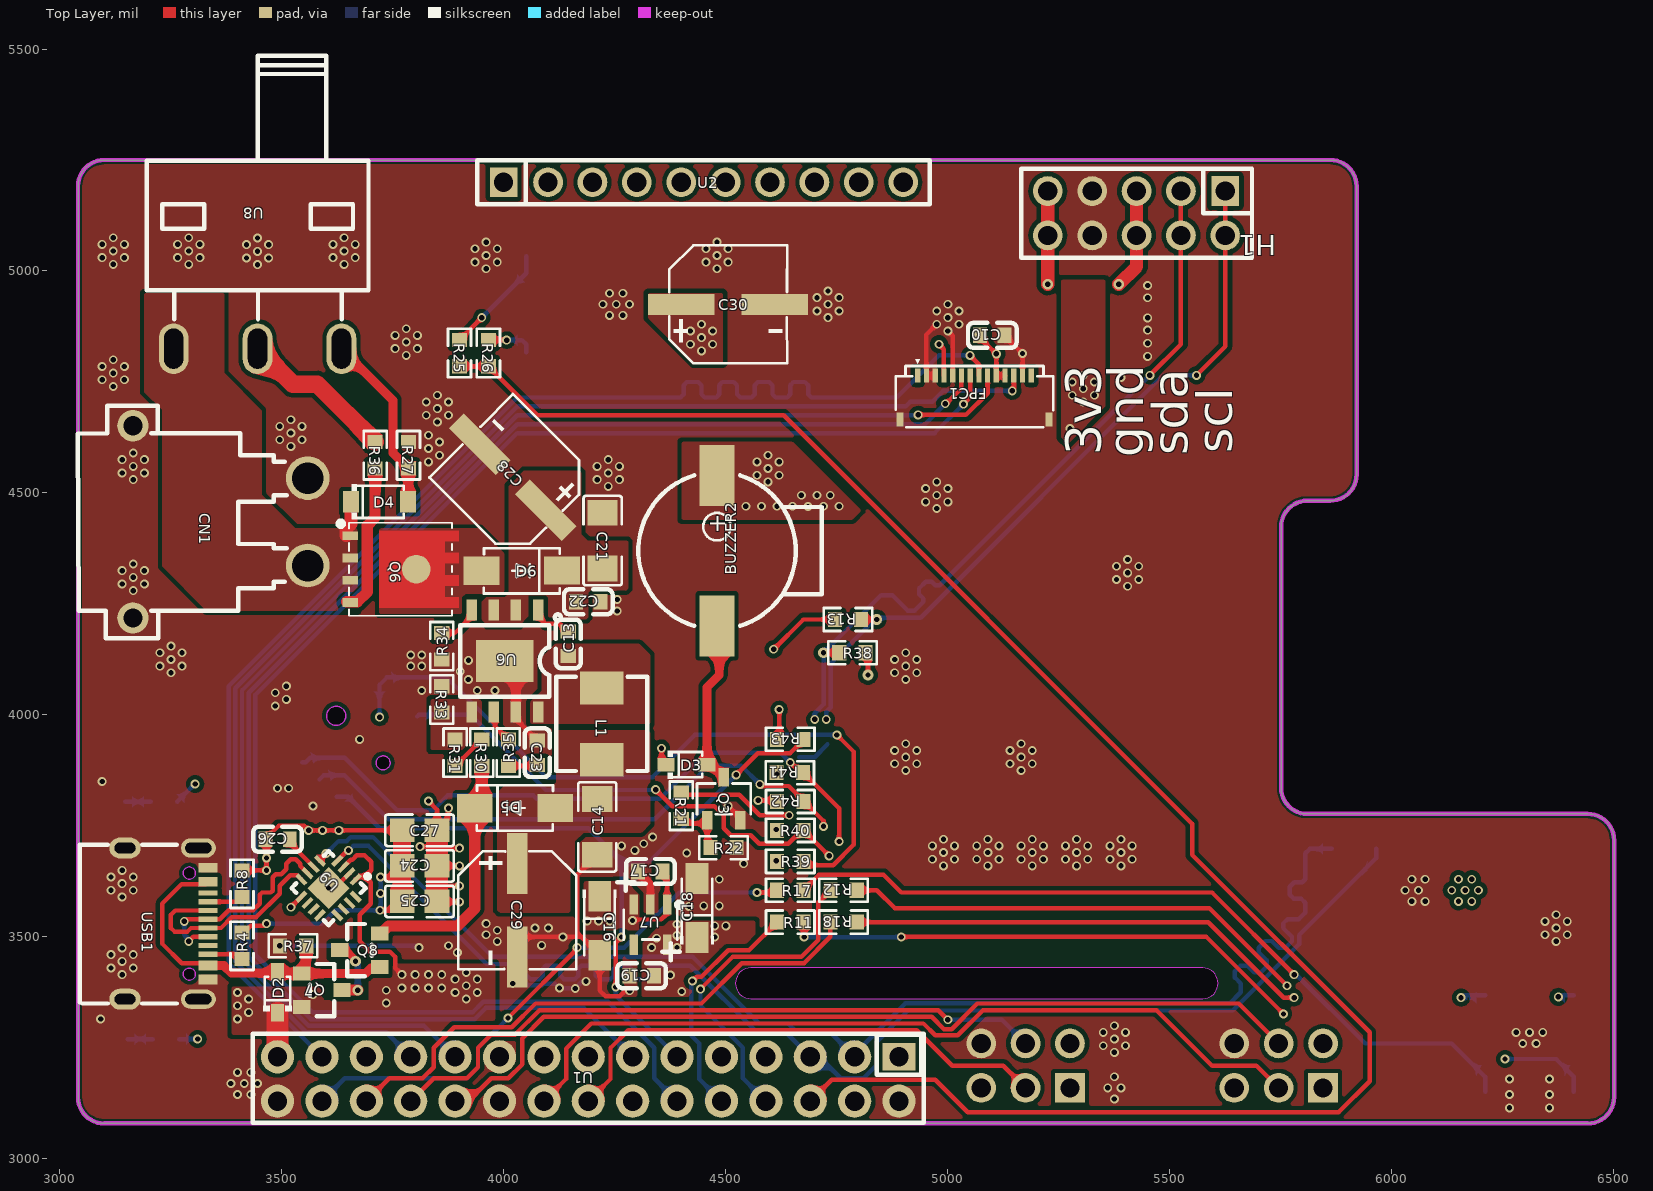
[diagram p0: Top Layer view]
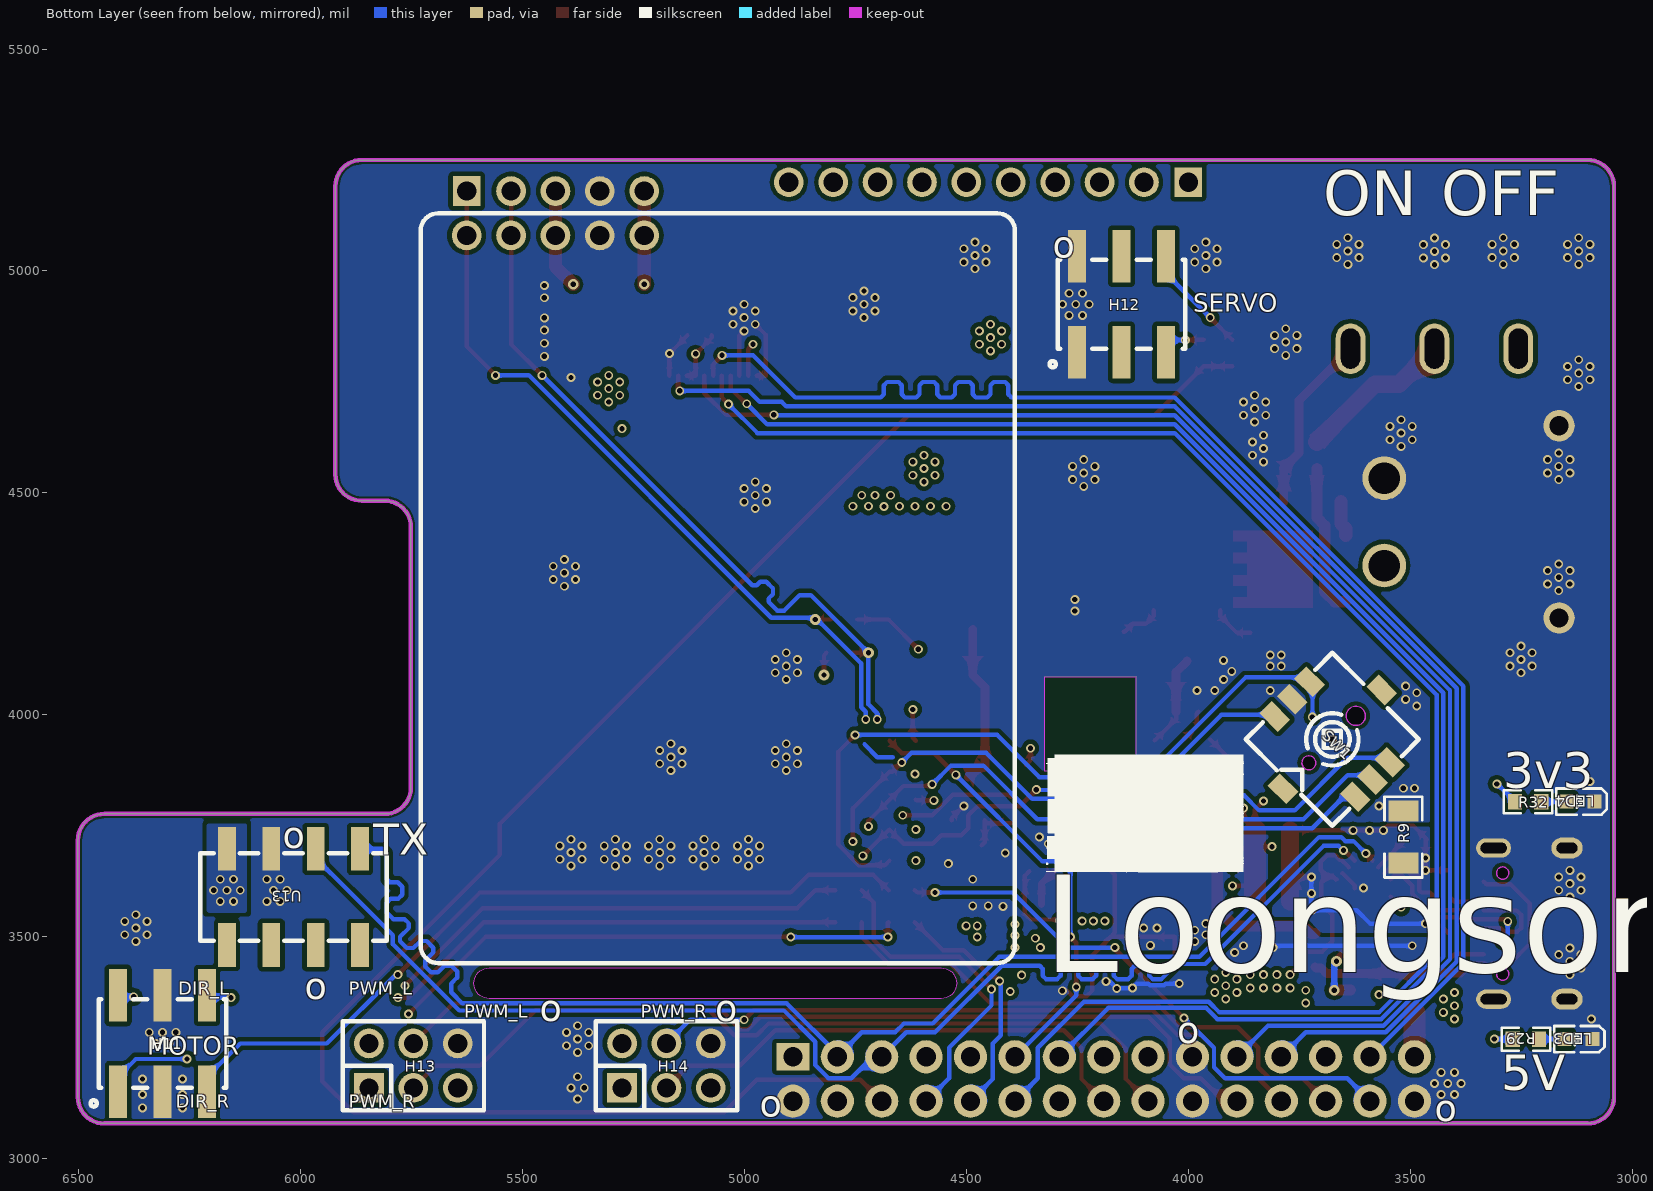
[diagram p1: Bottom Layer view, seen from below]
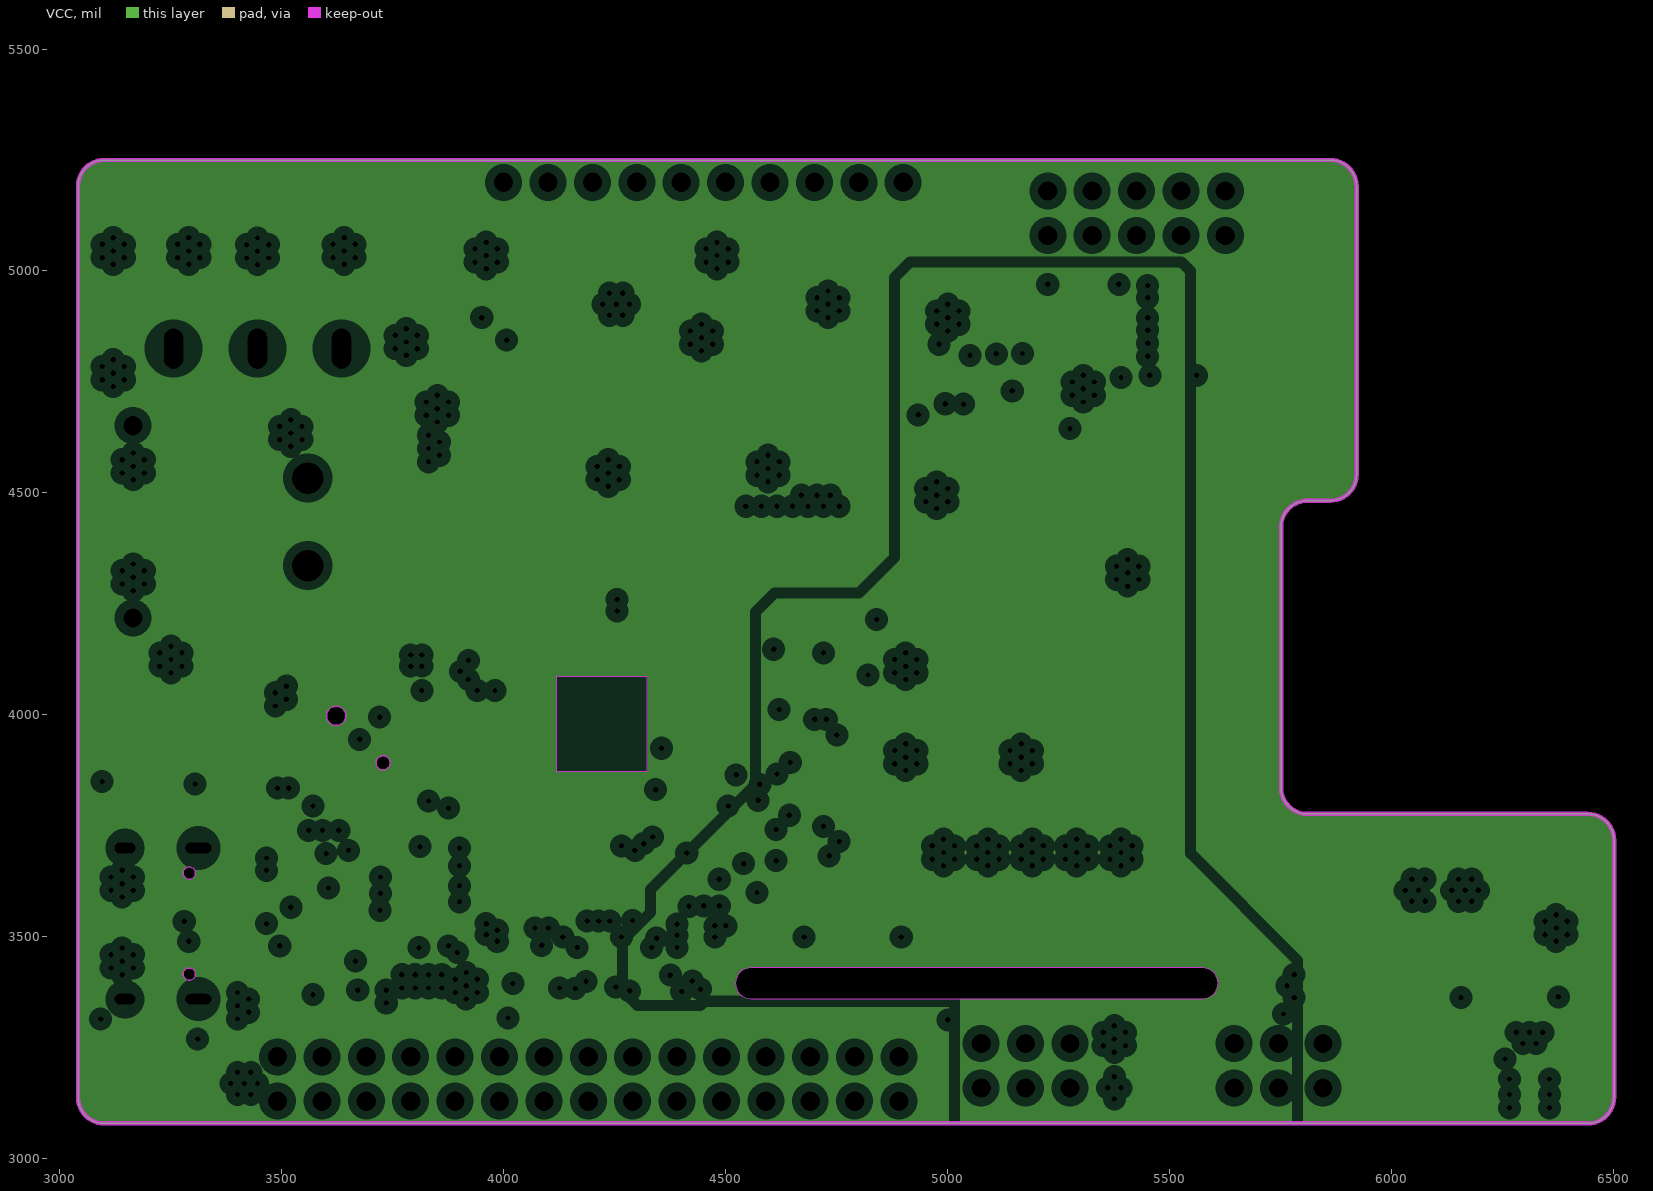
[diagram p2: VCC, clearances drawn from the general rule]
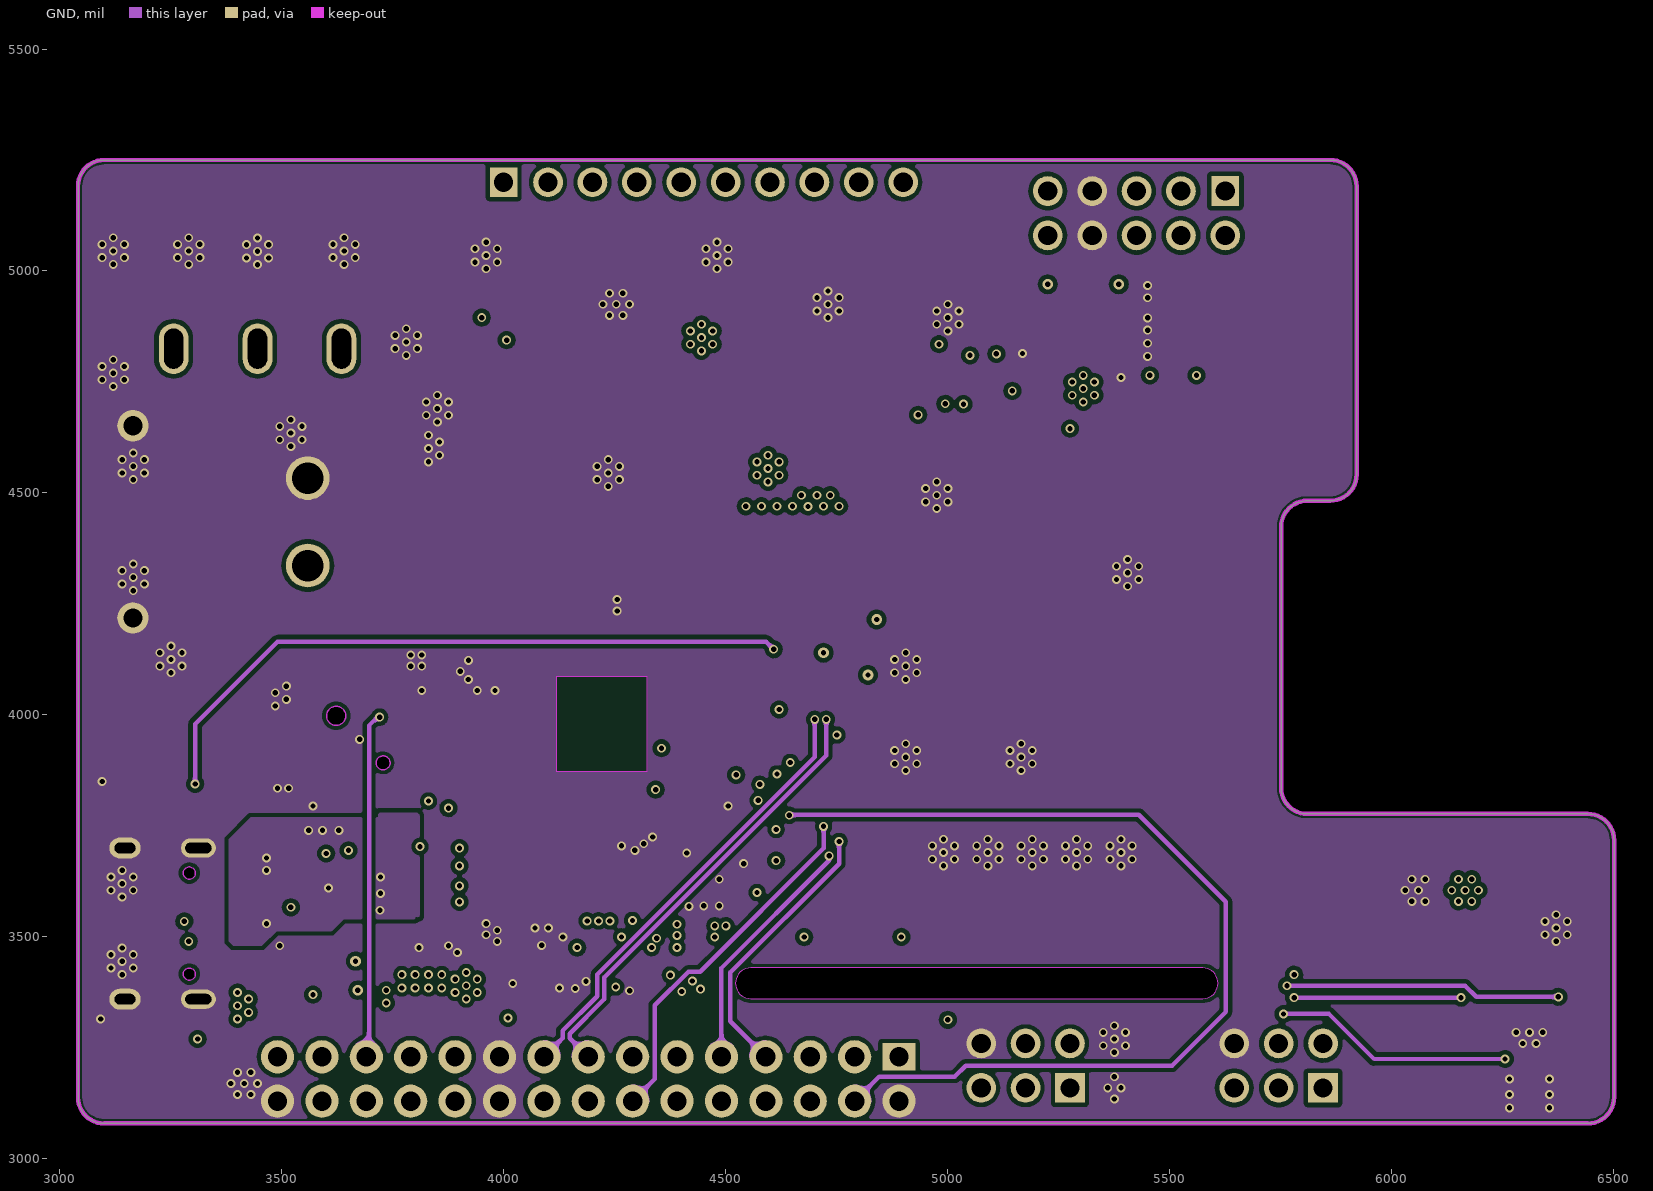
[diagram p3: GND]
# Altium PCB MISC51977.pcbdoc (part 1 of 4)
Units mil, origin at the board's own origin, x right, y up, seen from the top; angles counter-clockwise.
Board outline 3460 x 2170.19 mil, 4 copper layers (Top Layer, VCC, GND, Bottom Layer), stack 62.447 mil thick; 74 components, 60 nets, 282 pads, 462 vias.

## Layer stack, top to bottom
Top Layer: signal copper 1.378
Dielectric1: surface 8.283, 7628 RC49% 8.6mil, Dk 0
VCC: plane copper 0.598
Dielectric2: surface 41.929, 1.1mm H/HOZ Copper, Dk 0
GND: signal copper 0.598
Dielectric3: surface 8.283, 7628 RC49% 8.6mil, Dk 0
Bottom Layer: signal copper 1.378

## Board outline
3040.6,5190.94 3040.6,3138.86 ccw(c3099.66,3138.86) 3099.66,3079.81 6441.54,3079.81 ccw(c6441.54,3138.86) 6500.6,3138.86 6500.6,3717.98 ccw(c6441.54,3717.98) 6441.54,3777.04 5809.66,3777.04 cw(c5809.66,3836.09) 5750.6,3836.09 5750.6,4423.44 cw(c5809.66,4423.44) 5809.66,4482.5 5861.54,4482.5 ccw(c5861.54,4541.56) 5920.6,4541.56 5920.6,5190.94 ccw(c5861.54,5190.94) 5861.54,5250 3099.66,5250 ccw(c3099.66,5190.94)
cut-out: 4555.79,3430 ccw(c4555.79,3395.63) 4521.42,3395.63 ccw(c4555.79,3395.63) 4555.79,3361.26 5574.41,3361.26 ccw(c5574.41,3395.63) 5608.78,3395.63 ccw(c5574.41,3395.63) 5574.41,3430

## Design rules (kind name [scope] priority, off if disabled: settings)
BoardOutlineClearance copperThickness2oz_1 [All] p2 off: genericclearance=7.99 ignorepadtopadclearanceinfootprint=FALSE except(0: Arc-SplitContinuation Track-SplitContinuation SMDPad-SplitContinuation THPad-SplitContinuation Via-SplitContinuation Fill-SplitContinuation Region-SplitContinuation Poly-SplitContinuation Text-SplitContinuation Hole-SplitContinuation; 5.98: Arc-CutoutEdge Track-CutoutEdge SMDPad-CutoutEdge THPad-CutoutEdge Via-CutoutEdge Text-CutoutEdge; 6.89: Hole-OutlineEdge Hole-CutoutEdge; 10: Poly-OutlineEdge Poly-CutoutEdge; 11.81: Arc-OutlineEdge Track-OutlineEdge SMDPad-OutlineEdge THPad-OutlineEdge Via-OutlineEdge Fill-OutlineEdge Region-OutlineEdge Text-OutlineEdge Fill-CutoutEdge Region-CutoutEdge)
BoardOutlineClearance Plane_innerPlane_1 [All] p4 off: genericclearance=4.02 ignorepadtopadclearanceinfootprint=FALSE except(0: Arc-SplitContinuation Track-SplitContinuation SMDPad-SplitContinuation THPad-SplitContinuation Via-SplitContinuation Fill-SplitContinuation Region-SplitContinuation Poly-SplitContinuation Text-SplitContinuation Hole-SplitContinuation; 5.98: Arc-CutoutEdge Track-CutoutEdge SMDPad-CutoutEdge THPad-CutoutEdge Via-CutoutEdge Text-CutoutEdge; 6.89: Hole-OutlineEdge Hole-CutoutEdge; 10: Poly-OutlineEdge Poly-CutoutEdge; 11.81: Arc-OutlineEdge Track-OutlineEdge SMDPad-OutlineEdge THPad-OutlineEdge Via-OutlineEdge Fill-OutlineEdge Region-OutlineEdge Text-OutlineEdge Fill-CutoutEdge Region-CutoutEdge)
BoardOutlineClearance Copper_copperRegion_1 [All] p6 off: genericclearance=4.02 ignorepadtopadclearanceinfootprint=FALSE except(0: Arc-SplitContinuation Track-SplitContinuation SMDPad-SplitContinuation THPad-SplitContinuation Via-SplitContinuation Fill-SplitContinuation Region-SplitContinuation Poly-SplitContinuation Text-SplitContinuation Hole-SplitContinuation; 5.98: Arc-CutoutEdge Track-CutoutEdge SMDPad-CutoutEdge THPad-CutoutEdge Via-CutoutEdge Text-CutoutEdge; 6.89: Hole-OutlineEdge Hole-CutoutEdge; 10: Poly-OutlineEdge Poly-CutoutEdge; 11.81: Arc-OutlineEdge Track-OutlineEdge SMDPad-OutlineEdge THPad-OutlineEdge Via-OutlineEdge Fill-OutlineEdge Region-OutlineEdge Text-OutlineEdge Fill-CutoutEdge Region-CutoutEdge)
BoardOutlineClearance copperThickness1oz_1 [All] p8: genericclearance=4.02 ignorepadtopadclearanceinfootprint=FALSE except(0: Arc-SplitContinuation Track-SplitContinuation SMDPad-SplitContinuation THPad-SplitContinuation Via-SplitContinuation Fill-SplitContinuation Region-SplitContinuation Poly-SplitContinuation Text-SplitContinuation Hole-SplitContinuation; 5.98: Arc-CutoutEdge Track-CutoutEdge SMDPad-CutoutEdge THPad-CutoutEdge Via-CutoutEdge Text-CutoutEdge; 6.89: Hole-OutlineEdge Hole-CutoutEdge; 10: Poly-OutlineEdge Poly-CutoutEdge; 11.81: Arc-OutlineEdge Track-OutlineEdge SMDPad-OutlineEdge THPad-OutlineEdge Via-OutlineEdge Fill-OutlineEdge Region-OutlineEdge Text-OutlineEdge Fill-CutoutEdge Region-CutoutEdge)
Clearance copperThickness2oz [All] p1 off: gap=7.99 ignorepadtopadclearanceinfootprint=FALSE except(5.98: SMDPad-Track SMDPad-SMDPad THPad-Track SMDPad-THPad THPad-THPad Track-Via SMDPad-Via THPad-Via Via-Via Fill-SMDPad Region-SMDPad Fill-THPad Region-THPad Fill-Via Region-Via Fill-Fill Fill-Region Region-Region Arc-Track Arc-SMDPad Arc-THPad Arc-Via Fill-Arc Region-Arc Arc-Arc Text-Track SMDPad-Text Text-THPad Text-Via Fill-Text Region-Text Arc-Text Text-Text; 6.89: Hole-Track Hole-SMDPad Hole-THPad Hole-Via Fill-Hole Region-Hole Hole-Arc Hole-Text; 10: Poly-Track Poly-SMDPad Poly-THPad Poly-Via Poly-Fill Poly-Region Poly-Poly Poly-Arc Poly-Text Poly-Hole; 11.81: Fill-Track Region-Track)
Clearance Plane_innerPlane [All] p3 off: gap=4.02 ignorepadtopadclearanceinfootprint=FALSE except(5.98: SMDPad-Track SMDPad-SMDPad THPad-Track SMDPad-THPad THPad-THPad Track-Via SMDPad-Via THPad-Via Via-Via Fill-SMDPad Region-SMDPad Fill-THPad Region-THPad Fill-Via Region-Via Fill-Fill Fill-Region Region-Region Arc-Track Arc-SMDPad Arc-THPad Arc-Via Fill-Arc Region-Arc Arc-Arc Text-Track SMDPad-Text Text-THPad Text-Via Fill-Text Region-Text Arc-Text Text-Text; 6.89: Hole-Track Hole-SMDPad Hole-THPad Hole-Via Fill-Hole Region-Hole Hole-Arc Hole-Text; 10: Poly-Track Poly-SMDPad Poly-THPad Poly-Via Poly-Fill Poly-Region Poly-Poly Poly-Arc Poly-Text Poly-Hole; 11.81: Fill-Track Region-Track)
Clearance Copper_copperRegion [All] p5 off: gap=4.02 ignorepadtopadclearanceinfootprint=FALSE except(5.98: SMDPad-Track SMDPad-SMDPad THPad-Track SMDPad-THPad THPad-THPad Track-Via SMDPad-Via THPad-Via Via-Via Fill-SMDPad Region-SMDPad Fill-THPad Region-THPad Fill-Via Region-Via Fill-Fill Fill-Region Region-Region Arc-Track Arc-SMDPad Arc-THPad Arc-Via Fill-Arc Region-Arc Arc-Arc Text-Track SMDPad-Text Text-THPad Text-Via Fill-Text Region-Text Arc-Text Text-Text; 6.89: Hole-Track Hole-SMDPad Hole-THPad Hole-Via Fill-Hole Region-Hole Hole-Arc Hole-Text; 10: Poly-Track Poly-SMDPad Poly-THPad Poly-Via Poly-Fill Poly-Region Poly-Poly Poly-Arc Poly-Text Poly-Hole; 11.81: Fill-Track Region-Track)
Clearance copperThickness1oz [All] p7: gap=4.02 ignorepadtopadclearanceinfootprint=FALSE except(5.98: SMDPad-Track SMDPad-SMDPad THPad-Track SMDPad-THPad THPad-THPad Track-Via SMDPad-Via THPad-Via Via-Via Fill-SMDPad Region-SMDPad Fill-THPad Region-THPad Fill-Via Region-Via Fill-Fill Fill-Region Region-Region Arc-Track Arc-SMDPad Arc-THPad Arc-Via Fill-Arc Region-Arc Arc-Arc Text-Track SMDPad-Text Text-THPad Text-Via Fill-Text Region-Text Arc-Text Text-Text; 6.89: Hole-Track Hole-SMDPad Hole-THPad Hole-Via Fill-Hole Region-Hole Hole-Arc Hole-Text; 10: Poly-Track Poly-SMDPad Poly-THPad Poly-Via Poly-Fill Poly-Region Poly-Poly Poly-Arc Poly-Text Poly-Hole; 11.81: Fill-Track Region-Track)
DiffPairsRouting differentialPair [All] p1: maxlimit=6 minlimit=6 mostfreqgap=6 toplayer_minwidth=5 toplayer_prefwidth=10 toplayer_maxwidth=100 toplayer_mingap=6 toplayer_prefgap=6 toplayer_maxgap=6 midlayer1_minwidth=5 midlayer1_prefwidth=10 midlayer1_maxwidth=100 midlayer1_mingap=6 midlayer1_prefgap=6 midlayer1_maxgap=6 bottomlayer_minwidth=5 bottomlayer_prefwidth=10 bottomlayer_maxwidth=100 bottomlayer_mingap=6 bottomlayer_prefgap=6 bottomlayer_maxgap=6 maxuncoupledlength=10
HoleToHoleClearance otherClearance [All] p1: gap=11.81 allowstackedmicrovias=TRUE
Length netLength [All] p1: minlimit=0 maxlimit=0
PasteMaskExpansion pasteMaskExpansion [All] p1: expansion=0
PlaneConnect innerPlane [All] p1: planeconnectstyle=Direct reliefexpansion=20 reliefentries=4 reliefconductorwidth=10 reliefairgap=10
PolygonConnect copperRegion [All] p1: connectstyle=Direct reliefconductorwidth=10 reliefentries=4 polygonreliefangle="90 Angle" airgapwidth=10 via.connectstyle=Relief via.reliefconductorwidth=10 via.reliefentries=4 via.polygonreliefangle="90 Angle" via.airgapwidth=10
RoutingVias viaSize [All] p1: holewidth=12.01 width=24.02 viastyle="Through Hole" minholewidth=11.81 minwidth=19.68 maxholewidth=248.03 maxwidth=393.7
SolderMaskExpansion solderMaskExpansion [IsVia] p1: expansion=-1000 istentingtop=TRUE
SolderMaskExpansion solderMaskExpansion [All] p2: expansion=2.01 istentingtop=FALSE
Width copperThickness2oz_2 [All] p1 off: maxlimit=100 minlimit=8 preferedwidth=10
Width copperThickness1oz_2 [All] p2: maxlimit=100 minlimit=5 preferedwidth=10

## Components (designator, comment, footprint, x,y, rotation, side; value= is the part's Value field where it differs from the comment)
BUZZER2 "2.7kHz" BUZ-SMD_GSC9032RB 4480,4370 r90 top
C10 "100nF" C0603 5100,4855 r180 top
C13 "100nF" C0603 4145,4160 r90 top
C14 "47uF" C1206 4210.19,3747.83 r90 top
C16 "10uF" CAP-SMD_L3.2-W1.6-RD-C7171 4215.49,3525 r270 top
C17 "100nF" C0603 4330,3647.62 r180 top
C18 "10uF" CAP-SMD_L3.2-W1.6-RD-C7171 4435,3565 r90 top
C19 "100nF" C0603 4310,3412.62 r180 top
C21 "4.7uF" C1206 4222.3,4392.7 r270 top
C22 "100nF" C0603 4190,4255 r180 top
C23 "4.7nF" C0603 4075,3915 r270 top
C24 "1uF" C0805 3810,3660 r180 top
C25 "1uF" C0805 3810,3580 r180 top
C26 "100nF" C0603 3490,3720 r180 top
C27 "1uF" C0805 3810,3740 r0 top
C28 "100uF" CAP-SMD_BD6.3-L6.6-W6.6-FD-1 4020,4535 r135 top
C29 "220uF" CAP-SMD_BD6.3-L6.6-W6.6-LS7.3-FD-H7.7 4030,3560 r270 top
C30 "100uF" CAP-SMD_BD6.3-L6.6-W6.6-FD-1 4505,4925 r0 top
CN1 "XT30PW-M30.G.Y" CONN-TH_XT30PW-M 3361.27,4434.99 r270 top locked
D2 "1N5819WS" SOD-323_L1.8-W1.3-LS2.5-RD 3490,3375 r90 top
D3 "1N5819WS" SOD-323_L1.8-W1.3-LS2.5-RD 4411.22,3887.89 r0 top
D4 "BZT52C16" SOD-123_L2.7-W1.6-LS3.7-RD 3720,4480 r0 top
D5 "SS54" SMA_L4.3-W2.6-LS5.0-FD 4025,3790 r180 top
D6 "SS54" SMA_L4.3-W2.6-LS5.0-FD 4040,4325 r0 top
FPC1 "HC-FPC-05-09-14RLTAG" FPC-SMD_14P-P0.50_HC-FPC-05-09-14RLTAG 5060,4715 r180 top locked
H1 "" HDR-TH_10P-P2.54-V-F-R2-C5-S2.54 5425,5130 r180 top
H11 "HX PZ2.54-2x3P TP" HDR-SMD_6P-P2.54-V-M-R2-C3-LS7.2_M20-8760342 6310,3260 r180 bottom
H12 "HX PZ2.54-2x3P TP" HDR-SMD_6P-P2.54-V-M-R2-C3-LS7.2_M20-8760342 4150,4925 r180 bottom
H13 "PZ254V-12-6P" HDR-TH_6P-P2.54-V-M-R2-C3-S2.54 5745,3210 r180 bottom
H14 "PZ254V-12-6P" HDR-TH_6P-P2.54-V-M-R2-C3-S2.54 5175,3210 r180 bottom
L1 "4.7uH" IND-SMD_L5.4-W5.2_FXL0530 4220,3980 r270 top
LED3 "NCD0603R1" LED0603-RD_RED 3120.69,3270.05 r0 bottom
LED4 "NCD0603R1" LED0603-RD_RED 3115.69,3805.05 r0 bottom
Q3 "S8050" SOT-23-3_L2.9-W1.6-P1.90-LS2.8-BR 4495.26,3811.1 r270 top
Q6 "CJAC70P06" TDSON-8_L5.9-W5.2-P1.27-BL 3723.44,4328.38 r270 top
Q7 "AO3401A" SOT-23_L2.9-W1.3-P1.90-LS2.4-BR 3590,3380 r180 top
Q8 "AO3401A" SOT-23_L2.9-W1.3-P1.90-LS2.4-BR 3675,3470 r0 top
R4 "5.1kΩ" R0603 3410,3480 r90 top
R8 "5.1kΩ" R0603 3410,3619.53 r90 top
R9 "0Ω" R1206 3515,3725 r90 bottom
R11 "100Ω" R0603 4645,3533.35 r0 top
R12 "100Ω" R0603 4765,3605.05 r180 top
R13 "5.1kΩ" R0603 4775,4215 r180 top
R17 "100Ω" R0603 4645,3605.05 r0 top
R18 "100Ω" R0603 4765,3533.35 r180 top
R21 "1kΩ" R0603 4399.34,3795.46 r270 top
R22 "10kΩ" R0603 4494.58,3701.1 r0 top
R25 "100Ω" R0603 3900,4815 r270 top
R26 "100Ω" R0603 3965,4815 r270 top
R27 "10kΩ" R0603 3785,4585 r270 top
R29 "4.7kΩ" R0603 3239.07,3269.54 r0 bottom
R30 "51kΩ" R0603 3950,3915 r270 top
R31 "1.5kΩ" R0603 3890,3915 r270 top
R32 "2.7kΩ" R0603 3234.07,3804.54 r180 bottom
R33 "10kΩ" R0603 3860,4035 r270 top
R34 "200kΩ" R0603 3860,4155 r90 top
R35 "20kΩ" R0603 4010,3915 r90 top
R36 "10Ω" R0603 3710,4585 r270 top
R37 "10kΩ" R0603 3525,3480 r0 top
R38 "5.1kΩ" R0603 4785,4140 r0 top
R39 "10kΩ" R0603 4645,3670 r0 top
R40 "10kΩ" R0603 4645,3740 r0 top
R41 "10kΩ" R0603 4643.9,3870 r180 top
R42 "10kΩ" R0603 4645,3805 r180 top
R43 "10kΩ" R0603 4645,3945 r180 top
SW1 "7*7*5-6P-L WX" SW-SMD_8P-L7.0-W7.0-P1.40-LS7.4-TL 3675,3945 r225 bottom
U1 "2541FV-2x15P-B" HDR-TH_30P-P2.54-V-F-R2-C15-S2.54 4190,3180 r180 top locked
U2 "PM2.54-1*10" HDR-TH_10P-P2.54-V-F 4449.34,5199.86 r0 top locked
U6 "SCT2450STER" ESOP-8_L4.9-W3.9-P1.27-LS6.0-BL-EP 4002.11,4121.43 r180 top
U7 "RT9013-33GB" SOT-23-5_L3.0-W1.7-P0.95-LS2.8-BL 4330,3527.62 r180 top
U8 "SS12D10G6-WJ" SW-TH_3P-P4.80_HX-SS12D10G6-WJ 3445,4825 r180 top locked
U9 "CH343P" TQFN-16_L3.0-W3.0-P0.50-BL-EP1.7 3605,3610 r135 top
U13 "5BME8-08872-204-W0" CONN-SMD_5BME8-08872-204-W0 6015,3590 r0 bottom
USB1 "TYPE-C 16PIN 2MD(073)" USB-C-SMD_TYPE-C-6PIN-2MD-073 3240,3530 r270 top locked

## Footprints (in the part's own frame and the unit in brackets; to place one, negate y for a bottom-side part, rotate by r counter-clockwise, add the part's x,y. Pads: shape width x height; smd on the part's side, far side on the other; paste and mask are expansions set on the pad)
BUZ-SMD_GSC9032RB [mm]
  rect 3.5x2 smd: 1(4.3,0) 2(-4.3,0)
  silkscreen extent -4.3,-6 4.3,4.5
C0603 [mm]
  rect 0.8x0.9 smd: 1(-0.7,0) 2(0.7,0)
  silkscreen extent -1.39,-0.71 1.39,0.71
C0805 [mm]
  rect 1.41x1.35 smd paste-100 mask+0.051: 1(-1,0) 2(1,0)
  silkscreen extent -1.96,-0.9 1.96,0.9
C1206 [mm]
  rect 1.485x1.728 smd paste-100 mask+0.051: 1(-1.593,0) 2(1.593,0)
  silkscreen extent -2.56,-1.09 2.56,1.09
CAP-SMD_BD6.3-L6.6-W6.6-FD-1 [mm]
  rect 3.8x1.2 smd: 1(-2.67,0) 2(2.67,0)
  silkscreen extent -3.38,-3.38 3.38,3.38
CAP-SMD_BD6.3-L6.6-W6.6-LS7.3-FD-H7.7 [mm]
  rect 3.5x1.2 smd: 1(-2.67,0) 2(2.67,0)
  silkscreen extent -3.38,-3.38 3.38,3.38
CAP-SMD_L3.2-W1.6-RD-C7171 [mil]
  rect 69.19x51.02 smd: 1(-66.39,0) 2(66.39,0)
  silkscreen extent -118,-37 66,79
CONN-SMD_5BME8-08872-204-W0 [mm]
  rect 1.02x2.5 smd paste+0 mask+0.05: 1(-3.81,-2.75) 2(-3.81,2.75) 3(-1.27,-2.75) 4(-1.27,2.75) 5(1.27,-2.75) 6(1.27,2.75) 7(3.81,-2.75) 8(3.81,2.75)
  silkscreen extent -5.33,-2.5 5.33,2.5
CONN-TH_XT30PW-M [mm]
  round 2.5 hole 1.8: 1(-2.5,5) 2(2.5,5)
  round 1.8 hole 1.1: 3(5.5,-5) 4(-5.5,-5)
  silkscreen extent -6.65,-8.15 6.65,3.81
ESOP-8_L4.9-W3.9-P1.27-LS6.0-BL-EP [mm]
  rect 0.6x1.2 smd: 1(-1.905,-2.908) 2(-0.635,-2.908) 3(0.635,-2.908) 4(1.905,-2.908) 5(1.905,2.908) 6(0.635,2.908) 7(-0.635,2.908) 8(-1.905,2.908)
  rect 3.3x2.4 smd: 9(0,0)
  silkscreen extent -3.2,-2.67 2.55,2.05
FPC-SMD_14P-P0.50_HC-FPC-05-09-14RLTAG [mm]
  rect 0.3x0.8 smd paste+0 mask+0.05: 1(3.25,-1.25) 2(2.75,-1.25) 3(2.25,-1.25) 4(1.75,-1.25) 5(1.25,-1.25) 6(0.75,-1.25) 7(0.25,-1.25) 8(-0.25,-1.25) 9(-0.75,-1.25) 10(-1.25,-1.25) 11(-1.75,-1.25) 12(-2.25,-1.25) 13(-2.75,-1.25) 14(-3.25,-1.25)
  rect 0.4x0.8 smd paste+0 mask+0.05: 15(-4.25,1.25) 16(4.25,1.25)
  silkscreen extent -4.51,-2.18 4.51,1.71
HDR-SMD_6P-P2.54-V-M-R2-C3-LS7.2_M20-8760342 [mm]
  rect 1.02x3 smd: 1(-2.54,-2.75) 2(-2.54,2.75) 3(0,-2.75) 4(0,2.75) 5(2.54,-2.75) 6(2.54,2.75)
  silkscreen extent -4.12,-3.61 3.66,2.54
HDR-TH_6P-P2.54-V-M-R2-C3-S2.54 [mm]
  rect 1.7x1.7 hole 1.1: 1(-2.54,-1.27)
  round 1.7 hole 1.1: 2(-2.54,1.27) 3(0,-1.27) 4(0,1.27) 5(2.54,-1.27) 6(2.54,1.27)
  silkscreen extent -4.04,-2.54 4.04,2.54
HDR-TH_10P-P2.54-V-F [mm]
  rect 1.575x1.7 hole 1.1: 1(-11.43,0)
  round 1.7 hole 1.1: 2(-8.89,0) 3(-6.35,0) 4(-3.81,0) 5(-1.27,0) 6(1.27,0) 7(3.81,0) 8(6.35,0) 9(8.89,0) 10(11.43,0)
  silkscreen extent -12.95,-1.25 12.95,1.25
HDR-TH_10P-P2.54-V-F-R2-C5-S2.54 [mm]
  rect 1.575x1.7 hole 1.1: 1(-5.08,-1.27)
  round 1.7 hole 1.1: 2(-5.08,1.27) 3(-2.54,-1.27) 4(-2.54,1.27) 5(0,-1.27) 6(0,1.27) 7(2.54,-1.27) 8(2.54,1.27) 9(5.08,-1.27) 10(5.08,1.27)
  silkscreen extent -6.6,-2.54 6.6,2.54
HDR-TH_30P-P2.54-V-F-R2-C15-S2.54 [mm]
  rect 1.9x1.575 hole 1.1: 1(-17.78,-1.27)
  round 1.9 hole 1.1: 2(-17.78,1.27) 3(-15.24,-1.27) 4(-15.24,1.27) 5(-12.7,-1.27) 6(-12.7,1.27) 7(-10.16,-1.27) 8(-10.16,1.27) 9(-7.62,-1.27) 10(-7.62,1.27) 11(-5.08,-1.27) 12(-5.08,1.27) 13(-2.54,-1.27) 14(-2.54,1.27) 15(0,-1.27) 16(0,1.27) 17(2.54,-1.27) 18(2.54,1.27) 19(5.08,-1.27) 20(5.08,1.27) 21(7.62,-1.27) 22(7.62,1.27) 23(10.16,-1.27) 24(10.16,1.27) 25(12.7,-1.27) 26(12.7,1.27) 27(15.24,-1.27) 28(15.24,1.27) 29(17.78,-1.27) 30(17.78,1.27)
  silkscreen extent -19.2,-2.6 19.2,2.5
IND-SMD_L5.4-W5.2_FXL0530 [mm]
  rect 1.9x2.5 smd: 1(-2.05,0) 2(2.05,0)
  silkscreen extent -2.7,-2.6 2.7,2.6
LED0603-RD_RED [mm]
  rect 0.8x0.8 smd: 1(-0.8,-0.003) 2(0.8,0.003)
  silkscreen extent -1.49,-0.75 1.39,0.76
R0603 [mil]
  rect 31.75x34.02 smd paste-3937.01 mask+2: 1(-29.66,0) 2(29.66,0)
  silkscreen extent -55,-26 55,26
R1206 [mil]
  rect 47.54x66.97 smd paste-3937.01 mask+2: 1(-58.22,0) 2(58.22,0)
  silkscreen extent -91,-42 91,42
SMA_L4.3-W2.6-LS5.0-FD [mm]
  rect 2.046x1.62 smd: 1(-2.304,-0.009) 2(2.304,0.009)
  silkscreen extent -2.17,-1.32 2.19,1.29
SOD-123_L2.7-W1.6-LS3.7-RD [mm]
  rect 0.91x1.22 smd: 1(-1.635,0) 2(1.635,0)
  silkscreen extent -1.6,-1 1.38,1
SOD-323_L1.8-W1.3-LS2.5-RD [mm]
  rect 1x0.75 smd: 1(-1.173,0) 2(1.173,0)
  silkscreen extent -1.08,-0.8 0.9,0.8
SOT-23-3_L2.9-W1.6-P1.90-LS2.8-BR [mm]
  rect 1.07x0.6 smd: 1(1.235,-0.95) 2(1.235,0.95) 3(-1.235,0)
  silkscreen extent -0.88,-1.54 0.88,1.54
SOT-23-5_L3.0-W1.7-P0.95-LS2.8-BL [mm]
  rect 0.49x1.157 smd: 1(-0.95,-1.154) 2(0,-1.154) 3(0.95,-1.154)
  rect 0.49x1.175 smd: 4(0.95,1.154) 5(-0.95,1.154)
  silkscreen extent -1.8,-1.29 1.53,0.85
SOT-23_L2.9-W1.3-P1.90-LS2.4-BR [mm]
  rect 1x0.8 smd: 1(1.15,-0.95) 2(1.15,0.95) 3(-1.15,0)
  silkscreen extent -0.7,-1.5 0.7,1.5
SW-SMD_8P-L7.0-W7.0-P1.40-LS7.4-TL [mm]
  rect 1.5x1 smd paste+0 mask+0.05: 1(-3.25,1.4) 2(-3.25,0) 3(-3.25,-1.4) 4(3.25,-1.4) 5(3.25,0) 6(3.25,1.4) 7(0,4) 8(0,-4)
  Board Outline Layer circle w0.003: c0,1.9 r0.55
  Board Outline Layer circle w0.003: c0,-1.9 r0.4
  Board Outline Layer region: -0.389,1.511 -0.182,1.381 0.061,1.353 0.292,1.434 0.466,1.607 0.546,1.838 0.519,2.082 0.389,2.289 0.389,2.289 0.182,2.419 -0.062,2.446 -0.293,2.366 -0.466,2.192 -0.547,1.961 -0.519,1.718 -0.389,1.511
  Board Outline Layer region: -0.389,1.511 -0.311,1.446 -0.222,1.397 -0.126,1.364 -0.026,1.35 0.076,1.355 0.175,1.378 0.268,1.419 0.351,1.477 0.423,1.548 0.48,1.632 0.521,1.725 0.545,1.824 0.549,1.925 0.535,2.026 0.503,2.122 0.454,2.211 0.389,2.289 0.311,2.354 0.222,2.403 0.126,2.435 0.025,2.449 -0.076,2.445 -0.175,2.421 -0.268,2.38 -0.351,2.323 -0.423,2.251 -0.481,2.168 -0.522,2.075 -0.545,1.976 -0.55,1.874 -0.536,1.774 -0.503,1.678 -0.454,1.589
  Board Outline Layer region: -0.283,-2.183 -0.132,-2.278 0.045,-2.297 0.213,-2.239 0.339,-2.113 0.397,-1.945 0.377,-1.768 0.283,-1.617 0.283,-1.617 0.132,-1.522 -0.045,-1.502 -0.213,-1.561 -0.339,-1.687 -0.398,-1.855 -0.378,-2.032 -0.283,-2.183
  Board Outline Layer region: -0.283,-2.183 -0.213,-2.239 -0.132,-2.278 -0.045,-2.297 0.045,-2.297 0.132,-2.278 0.213,-2.239 0.283,-2.183 0.339,-2.113 0.377,-2.032 0.397,-1.945 0.397,-1.855 0.377,-1.768 0.339,-1.687 0.283,-1.617 0.213,-1.561 0.132,-1.522 0.045,-1.502 -0.045,-1.502 -0.132,-1.522 -0.213,-1.561 -0.283,-1.617 -0.339,-1.687 -0.378,-1.768 -0.398,-1.855 -0.398,-1.945 -0.378,-2.032 -0.339,-2.113
  Multi-Layer board cut-out: -0.389,1.511 -0.182,1.381 0.061,1.353 0.292,1.434 0.466,1.607 0.546,1.838 0.519,2.082 0.389,2.289 0.389,2.289 0.182,2.419 -0.062,2.446 -0.293,2.366 -0.466,2.192 -0.547,1.961 -0.519,1.718 -0.389,1.511
  Multi-Layer board cut-out: -0.283,-2.183 -0.132,-2.278 0.045,-2.297 0.213,-2.239 0.339,-2.113 0.397,-1.945 0.377,-1.768 0.283,-1.617 0.283,-1.617 0.132,-1.522 -0.045,-1.502 -0.213,-1.561 -0.339,-1.687 -0.398,-1.855 -0.378,-2.032 -0.283,-2.183
  silkscreen extent -3.5,-3.5 3.5,3.5
SW-TH_3P-P4.80_HX-SS12D10G6-WJ [mm]
  oval 1.7x2.9 hole 1.1 slot 2.3 at 90 deg paste+0 mask+0.05: 1(-4.8,0) 2(0,0) 3(4.8,0)
  silkscreen extent -6.35,-16.75 6.35,-1.68
TDSON-8_L5.9-W5.2-P1.27-BL [mm]
  rect 0.5x0.9 smd paste-100 mask+0.05: 1(-1.905,-1.775) 2(-0.635,-1.775) 3(0.635,-1.775) 4(1.905,-1.775)
  round 1.638 smd: 5(0,2.012)
  Top Layer region: -2.205,-0.1 2.205,-0.1 2.205,4.45 1.605,4.45 1.605,3.65 0.935,3.65 0.935,4.45 0.335,4.45 0.335,3.65 -0.335,3.65 -0.335,4.45 -0.935,4.45 -0.935,3.65 -1.605,3.65 -1.605,4.45 -2.205,4.45
  silkscreen extent -2.75,-2.46 2.66,4.06
TQFN-16_L3.0-W3.0-P0.50-BL-EP1.7 [mm]
  rect 0.25x0.75 smd paste-100 mask+0.051: 1(-0.748,-1.45) 2(-0.249,-1.45) 3(0.252,-1.45) 4(0.751,-1.45) 9(0.75,1.45) 10(0.25,1.45) 11(-0.25,1.45) 12(-0.749,1.45)
  rect 0.75x0.25 smd paste-100 mask+0.051: 5(1.45,-0.75) 6(1.45,-0.25) 7(1.45,0.25) 8(1.45,0.75) 13(-1.45,0.75) 14(-1.45,0.25) 15(-1.45,-0.25) 16(-1.45,-0.75)
  rect 1.7x1.7 smd paste-100 mask+0.051: 17(0,0)
  silkscreen extent -1.5,-2.17 1.5,1.5
USB-C-SMD_TYPE-C-6PIN-2MD-073 [mm]
  rect 0.55x1.1 smd paste-100 mask+0.05: 1(-3.2,2.375) 2(-2.4,2.375) 11(2.4,2.375) 12(3.2,2.375)
  rect 0.3x1.1 smd paste-100 mask+0.05: 3(-1.75,2.375) 4(-1.25,2.375) 5(-0.75,2.375) 6(-0.25,2.375) 7(0.25,2.375) 8(0.75,2.375) 9(1.25,2.375) 10(1.75,2.375)
  oval 1.2x1.8 hole 0.6 slot 1.2 at 90 deg paste+0 mask+0.05: 13(-4.325,-2.375) 14(4.325,-2.375)
  oval 1.1x2 hole 0.6 slot 1.5 at 90 deg paste+0 mask+0.05: 13(-4.325,1.825) 14(4.325,1.825)
  Board Outline Layer circle w0.003: c-2.89,1.305 r0.35
  Board Outline Layer circle w0.003: c2.89,1.305 r0.35
  Board Outline Layer region: -2.89,1.655 -2.738,1.62 -2.616,1.523 -2.549,1.383 -2.549,1.227 -2.616,1.087 -2.738,0.99 -2.89,0.955 -2.89,0.955 -3.042,0.99 -3.164,1.087 -3.231,1.227 -3.231,1.383 -3.164,1.523 -3.042,1.62 -2.89,1.655
  Board Outline Layer region: -2.89,1.655 -2.812,1.646 -2.738,1.62 -2.672,1.579 -2.616,1.523 -2.575,1.457 -2.549,1.383 -2.54,1.305 -2.549,1.227 -2.575,1.153 -2.616,1.087 -2.672,1.031 -2.738,0.99 -2.812,0.964 -2.89,0.955 -2.968,0.964 -3.042,0.99 -3.108,1.031 -3.164,1.087 -3.205,1.153 -3.231,1.227 -3.24,1.305 -3.231,1.383 -3.205,1.457 -3.164,1.523 -3.108,1.579 -3.042,1.62 -2.968,1.646
  Board Outline Layer region: 2.89,1.655 3.042,1.62 3.164,1.523 3.231,1.383 3.231,1.227 3.164,1.087 3.042,0.99 2.89,0.955 2.89,0.955 2.738,0.99 2.616,1.087 2.549,1.227 2.549,1.383 2.616,1.523 2.738,1.62 2.89,1.655
  Board Outline Layer region: 2.89,1.655 2.968,1.646 3.042,1.62 3.108,1.579 3.164,1.523 3.205,1.457 3.231,1.383 3.24,1.305 3.231,1.227 3.205,1.153 3.164,1.087 3.108,1.031 3.042,0.99 2.968,0.964 2.89,0.955 2.812,0.964 2.738,0.99 2.672,1.031 2.616,1.087 2.575,1.153 2.549,1.227 2.54,1.305 2.549,1.383 2.575,1.457 2.616,1.523 2.672,1.579 2.738,1.62 2.812,1.646
  Multi-Layer board cut-out: -2.89,1.655 -2.738,1.62 -2.616,1.523 -2.549,1.383 -2.549,1.227 -2.616,1.087 -2.738,0.99 -2.89,0.955 -2.89,0.955 -3.042,0.99 -3.164,1.087 -3.231,1.227 -3.231,1.383 -3.164,1.523 -3.042,1.62 -2.89,1.655
  Multi-Layer board cut-out: 2.89,1.655 3.042,1.62 3.164,1.523 3.231,1.383 3.231,1.227 3.164,1.087 3.042,0.99 2.89,0.955 2.89,0.955 2.738,0.99 2.616,1.087 2.549,1.227 2.549,1.383 2.616,1.523 2.738,1.62 2.89,1.655
  silkscreen extent -4.5,-4.97 4.57,0.6

## Via types
v1: diameter 20, hole 12, Top Layer to Bottom Layer, 455 vias
v2: diameter 24.02, hole 12, Top Layer to Bottom Layer, 7 vias